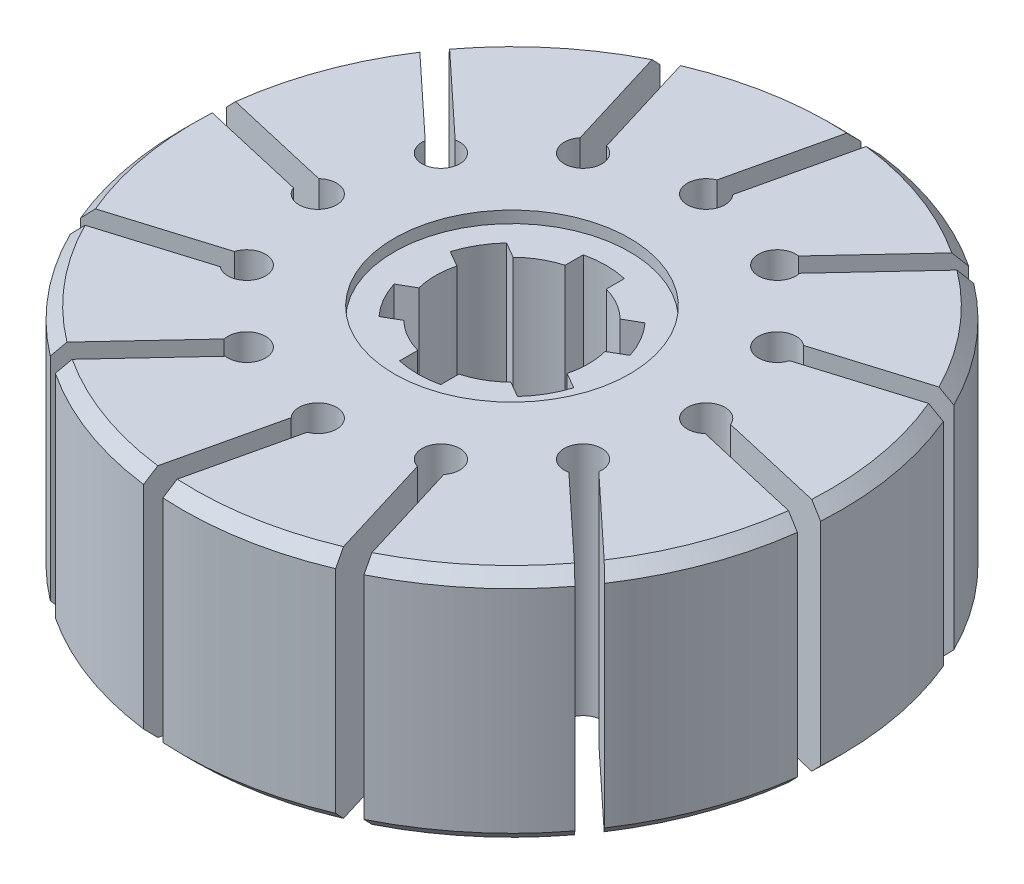
from build123d import *

# Parameters (mm, degrees)
SKETCH1_R           = 28
BOSS_EXTRUDE1_DEPTH = 20
SKETCH2_R           = 10
CUT_EXTRUDE1_DEPTH  = 1
CUT_EXTRUDE2_DEPTH  = 30
CUT_EXTRUDE3_START  = -1
SKETCH4_R           = 10
CUT_EXTRUDE3_DEPTH  = 1
SKETCH5_R           = 1.6
CUT_EXTRUDE4_DEPTH  = 80
CHAMFER1_SIZE       = 1
CUT_EXTRUDE5_DEPTH  = 80


with BuildPart() as part:
    # Sketch1 → Boss-Extrude1 (new body)
    with BuildSketch(Plane(origin=(0, 0, 0), x_dir=(1, 0, 0), z_dir=(0, 1, 0))):
        with Locations(Location((0, 0, 0), (0, 0, 270))):
            Circle(SKETCH1_R)
    extrude(amount=BOSS_EXTRUDE1_DEPTH)

    # Sketch2 → Cut-Extrude1 (cut)
    with BuildSketch(Plane(origin=(0, 20, 0), x_dir=(1, 0, 0), z_dir=(0, 1, 0))):
        with Locations(Location((0, 0, 0), (0, 0, 270))):
            Circle(SKETCH2_R)
    extrude(amount=-CUT_EXTRUDE1_DEPTH, mode=Mode.SUBTRACT)

    # Sketch3 → Cut-Extrude2 (cut)
    with BuildSketch(Plane(origin=(0, 19, 0), x_dir=(1, 0, 0), z_dir=(0, 1, 0))):
        with BuildLine():
            Line((-1.75, 7.806247498), (-1.75, 6.259992013))
            ThreePointArc((-1.75, 6.259992013), (-3.25, 5.629165125), (-4.546312111, 4.645540463))
            Line((-4.546312111, 4.645540463), (-5.885408641, 5.418668206))
            ThreePointArc((-5.885408641, 5.418668206), (-6.92820323, 4), (-7.635408641, 2.387579292))
            Line((-7.635408641, 2.387579292), (-6.296312111, 1.61445155))
            ThreePointArc((-6.296312111, 1.61445155), (-6.5, 0), (-6.296312111, -1.61445155))
            Line((-6.296312111, -1.61445155), (-7.635408641, -2.387579292))
            ThreePointArc((-7.635408641, -2.387579292), (-6.92820323, -4), (-5.885408641, -5.418668206))
            Line((-5.885408641, -5.418668206), (-4.546312111, -4.645540463))
            ThreePointArc((-4.546312111, -4.645540463), (-3.25, -5.629165125), (-1.75, -6.259992013))
            Line((-1.75, -6.259992013), (-1.75, -7.806247498))
            ThreePointArc((-1.75, -7.806247498), (0, -8), (1.75, -7.806247498))
            Line((1.75, -7.806247498), (1.75, -6.259992013))
            ThreePointArc((1.75, -6.259992013), (3.25, -5.629165125), (4.546312111, -4.645540463))
            Line((4.546312111, -4.645540463), (5.885408641, -5.418668206))
            ThreePointArc((5.885408641, -5.418668206), (6.92820323, -4), (7.635408641, -2.387579292))
            Line((7.635408641, -2.387579292), (6.296312111, -1.61445155))
            ThreePointArc((6.296312111, -1.61445155), (6.5, 0), (6.296312111, 1.61445155))
            Line((6.296312111, 1.61445155), (7.635408641, 2.387579292))
            ThreePointArc((7.635408641, 2.387579292), (6.92820323, 4), (5.885408641, 5.418668206))
            Line((5.885408641, 5.418668206), (4.546312111, 4.645540463))
            ThreePointArc((4.546312111, 4.645540463), (3.25, 5.629165125), (1.75, 6.259992013))
            Line((1.75, 6.259992013), (1.75, 7.806247498))
            ThreePointArc((1.75, 7.806247498), (0, 8), (-1.75, 7.806247498))
        make_face()
    extrude(amount=-CUT_EXTRUDE2_DEPTH, mode=Mode.SUBTRACT)

    # Sketch4 → Cut-Extrude3 (cut)
    with BuildSketch(Plane(origin=(0, 0, 0), x_dir=(-1, 0, 0), z_dir=(0, -1, 0)).offset(CUT_EXTRUDE3_START)):
        with Locations(Location((0, 0, 0), (0, 0, 270))):
            Circle(SKETCH4_R)
    extrude(amount=CUT_EXTRUDE3_DEPTH, mode=Mode.SUBTRACT)

    # Sketch5 → Cut-Extrude4 (cut)
    with BuildSketch(Plane(origin=(0, 20, 0), x_dir=(1, 0, 0), z_dir=(0, 1, 0))):
        with Locations(Location((0, 16.5, 0), (0, 0, 270))):
            Circle(SKETCH5_R)
        with Locations(Location((8.25, 14.289419162, 0), (0, 0, 270))):
            Circle(SKETCH5_R)
        with Locations(Location((14.289419162, 8.25, 0), (0, 0, 270))):
            Circle(SKETCH5_R)
        with Locations(Location((16.5, 0, 0), (0, 0, 270))):
            Circle(SKETCH5_R)
        with Locations(Location((14.289419162, -8.25, 0), (0, 0, 270))):
            Circle(SKETCH5_R)
        with Locations(Location((8.25, -14.289419162, 0), (0, 0, 270))):
            Circle(SKETCH5_R)
        with Locations(Location((0, -16.5, 0), (0, 0, 270))):
            Circle(SKETCH5_R)
        with Locations(Location((-8.25, -14.289419162, 0), (0, 0, 270))):
            Circle(SKETCH5_R)
        with Locations(Location((-14.289419162, -8.25, 0), (0, 0, 270))):
            Circle(SKETCH5_R)
        with Locations(Location((-16.5, 0, 0), (0, 0, 270))):
            Circle(SKETCH5_R)
        with Locations(Location((-14.289419162, 8.25, 0), (0, 0, 270))):
            Circle(SKETCH5_R)
        with Locations(Location((-8.25, 14.289419162, 0), (0, 0, 270))):
            Circle(SKETCH5_R)
    extrude(amount=-CUT_EXTRUDE4_DEPTH, mode=Mode.SUBTRACT)

    # Chamfer1
    chamfer1_edges = [part.edges().sort_by_distance(p)[0] for p in [
        (0, 0, -28),
        (0, 20, -28),
    ]]
    chamfer(chamfer1_edges, length=CHAMFER1_SIZE)

    # Sketch6 → Cut-Extrude5 (cut)
    with BuildSketch(Plane(origin=(0, 20, 0), x_dir=(1, 0, 0), z_dir=(0, 1, 0))):
        Polygon((0.876933058, 16.297544051), (4.195472987, 30.671719689), (2.44160687, 31.076631587), (-0.876933058, 16.702455949), align=None)
        Polygon((7.591781669, 14.903217686), (8.908218331, 13.675620638), (18.969246032, 24.464751935), (17.652809369, 25.692348984), align=None)
        Polygon((14.026284628, 9.11067428), (14.552553697, 7.38932572), (28.660224922, 11.702473657), (28.133955854, 13.423822218), align=None)
        Polygon((16.702455949, 0.876933058), (16.297544051, -0.876933058), (30.671719689, -4.195472987), (31.076631587, -2.44160687), align=None)
        Polygon((14.903217687, -7.591781669), (13.675620638, -8.908218331), (24.464751935, -18.969246032), (25.692348984, -17.652809369), align=None)
        Polygon((9.11067428, -14.026284628), (7.38932572, -14.552553697), (11.702473657, -28.660224922), (13.423822218, -28.133955854), align=None)
        Polygon((0.876933058, -16.702455949), (-0.876933058, -16.297544051), (-4.195472987, -30.671719689), (-2.44160687, -31.076631587), align=None)
        Polygon((-7.591781669, -14.903217686), (-8.908218331, -13.675620638), (-18.969246032, -24.464751935), (-17.652809369, -25.692348984), align=None)
        Polygon((-14.026284628, -9.11067428), (-14.552553697, -7.38932572), (-28.660224922, -11.702473657), (-28.133955854, -13.423822218), align=None)
        Polygon((-16.702455949, -0.876933058), (-16.297544051, 0.876933058), (-30.671719689, 4.195472987), (-31.076631587, 2.44160687), align=None)
        Polygon((-14.903217686, 7.591781669), (-13.675620638, 8.908218331), (-24.464751935, 18.969246032), (-25.692348984, 17.652809369), align=None)
        Polygon((-9.11067428, 14.026284628), (-7.38932572, 14.552553697), (-11.702473657, 28.660224922), (-13.423822218, 28.133955854), align=None)
    extrude(amount=-CUT_EXTRUDE5_DEPTH, mode=Mode.SUBTRACT)


solid = part.part
